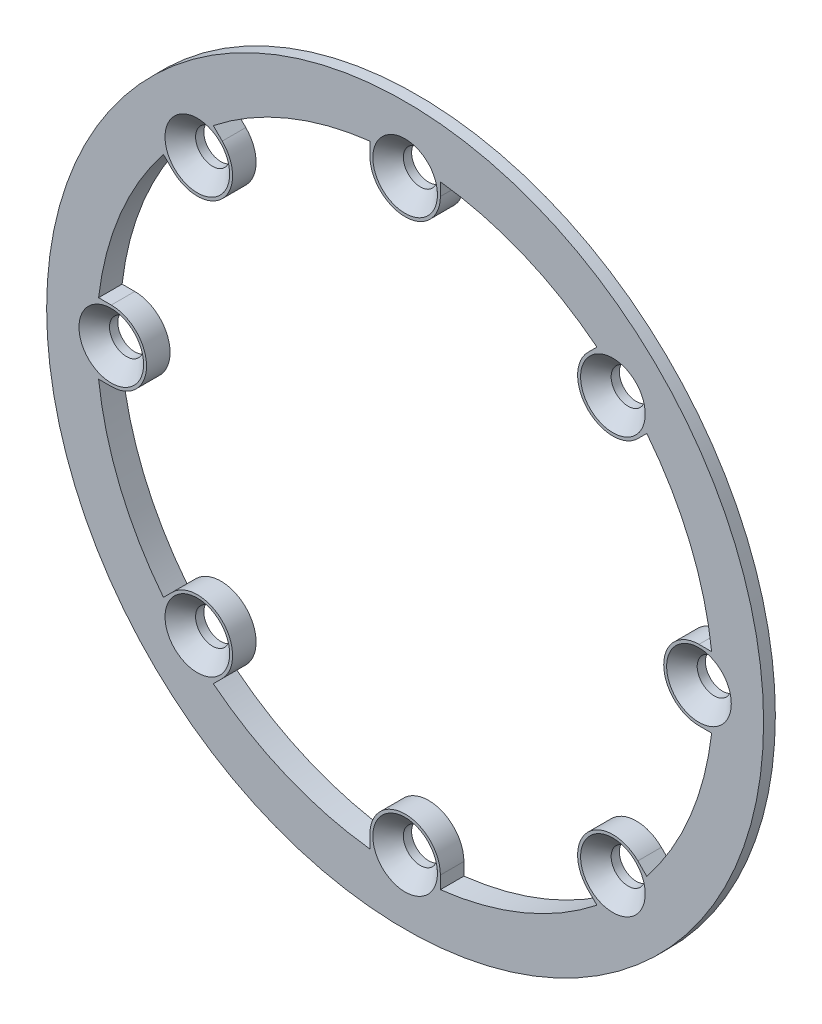
SolidWorks part; units mm, degrees
ref_plane "Front Plane" through (0, 0, 0) normal (0, 0, 1) x (1, 0, 0)
ref_plane "Top Plane" through (0, 0, 0) normal (0, 1, 0) x (1, 0, 0)
ref_plane "Right Plane" through (0, 0, 0) normal (1, 0, 0) x (0, 0, -1)
sketch "Sketch1" plane through (0, 0, 0) normal (0, 0, 1) x (1, 0, 0)
  circle A0 centre (0, 0) radius 26.25
  circle A1 centre (0, 0) radius 30.5
  dimension "D1" = 52.5
  dimension "D2" = 61
extrude "Boss-Extrude1" add sketch "Sketch1" along normal mid plane 2
chamfer "Chamfer1" distance 1.5 distance2 1 1 edges at (30.5, 0, -1)
sketch "Sketch4" plane through (0, 0, 1) normal (0, 0, 1) x (1, 0, 0)
  line L0 (-3, 25) -> (-3, 26.078)
  line L1 (3, 25) -> (3, 26.078)
  arc A0 (-3, 25) -> (3, 25) centre (0, 25) ccw
  circle A1 centre (0, 0) radius 26.25 construction
  arc A2 (3, 26.078) -> (-3, 26.078) centre (0, 0) ccw
  dimension "D1" = 6
  dimension "D2" = 25
extrude "Boss-Extrude2" add sketch "Sketch4" against normal up to surface (2 mm away) up to face at (29, 0, -1)
hole_wizard "CSK for M2.5 Countersunk Flat Head Screw2" positions "Sketch6" profile "Sketch5" countersink size "M2.5" standard "Iso" end condition through all
sketch "Sketch6" plane through (0, 0, 1) normal (0, 0, 1) x (1, 0, 0)
  point P0 (0, 25)
sketch "Sketch5" plane through (0, 25, 1) normal (1, 0, 0) x (0, -1, 0)
  line L0 (0, 0) -> (0, 2)
  line L1 (0, 2) -> (1.45, 2)
  line L2 (1.45, 2) -> (1.45, 1.3)
  line L3 (1.45, 1.3) -> (2.75, 0)
  line L5 (2.75, 0) -> (0, 0)
  line L6 (-1.45, 1.3) -> (-2.75, 0) construction
  line L11 (0, -6.35) -> (0, 107.95) construction
  dimension "通孔孔直径" = 2.9
  dimension "通孔孔深度" = 2
  dimension "近端锥形沉头孔直径" = 5.5
  dimension "近端锥形沉头孔角度" = 90
pattern_circular "CirPattern2" count 8 over 360 about axis through (0, 0, 0) along (0, 0, 1) of "Boss-Extrude2", "CSK for M2.5 Countersunk Flat Head Screw2"
